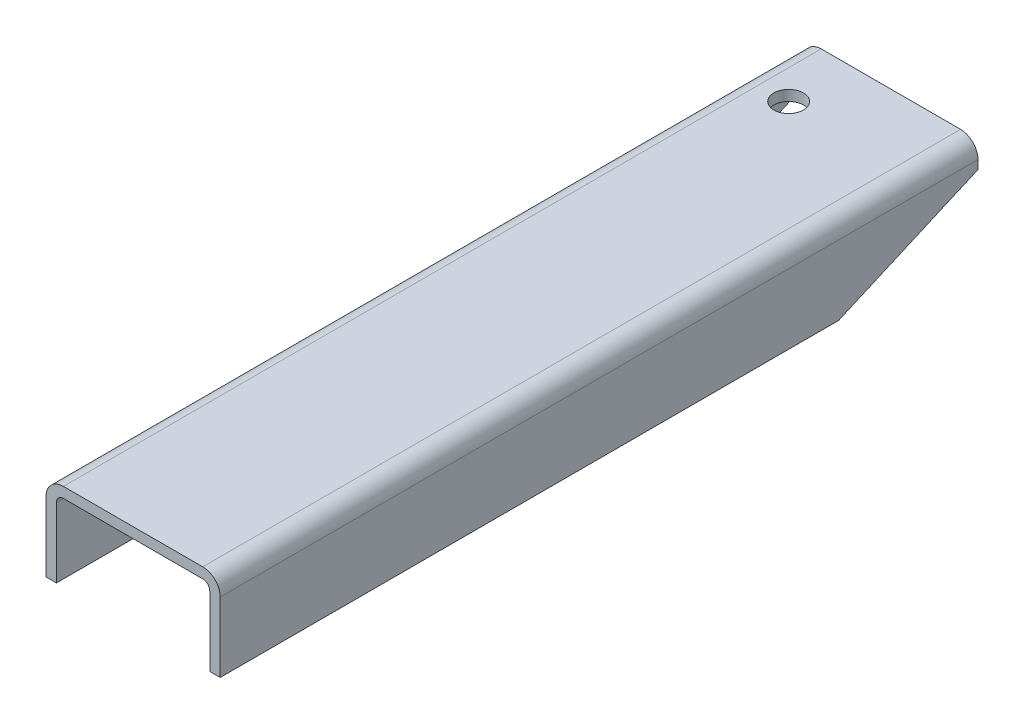
from build123d import *

# Parameters (mm, degrees)
BOSS_EXTRUDE1_DEPTH = 435
SKETCH2_R           = 8.5
CUT_EXTRUDE1_DEPTH  = 435
CUT_EXTRUDE2_DEPTH  = 435


with BuildPart() as part:
    # Sketch1 → Boss-Extrude1 (new body)
    with BuildSketch(Plane.XY):
        with BuildLine():
            Line((0, 0), (0, 40))
            ThreePointArc((0, 40), (2.928932188, 47.071067812), (10, 50))
            Line((10, 50), (90, 50))
            ThreePointArc((90, 50), (97.071067812, 47.071067812), (100, 40))
            Line((100, 40), (100, 0))
            Line((100, 0), (94, 0))
            Line((94, 0), (94, 40))
            ThreePointArc((94, 40), (92.828427125, 42.828427125), (90, 44))
            Line((90, 44), (10, 44))
            ThreePointArc((10, 44), (7.171572875, 42.828427125), (6, 40))
            Line((6, 40), (6, 0))
            Line((6, 0), (0, 0))
        make_face()
    extrude(amount=BOSS_EXTRUDE1_DEPTH)

    # Sketch2 → Cut-Extrude1 (cut)
    with BuildSketch(Plane(origin=(0, 50, 0), x_dir=(1, 0, 0), z_dir=(0, 1, 0))):
        with Locations(Location((26.8, -35.5, 0), (0, 0, 270))):
            Circle(SKETCH2_R)
    extrude(amount=-CUT_EXTRUDE1_DEPTH, mode=Mode.SUBTRACT)

    # Sketch3 → Cut-Extrude2 (cut)
    with BuildSketch(Plane(origin=(100, 0, 0), x_dir=(0, 0, -1), z_dir=(1, 0, 0))):
        Polygon((-80, 0), (0, 35), (0, 0), align=None)
    extrude(amount=-CUT_EXTRUDE2_DEPTH, mode=Mode.SUBTRACT)


solid = part.part
